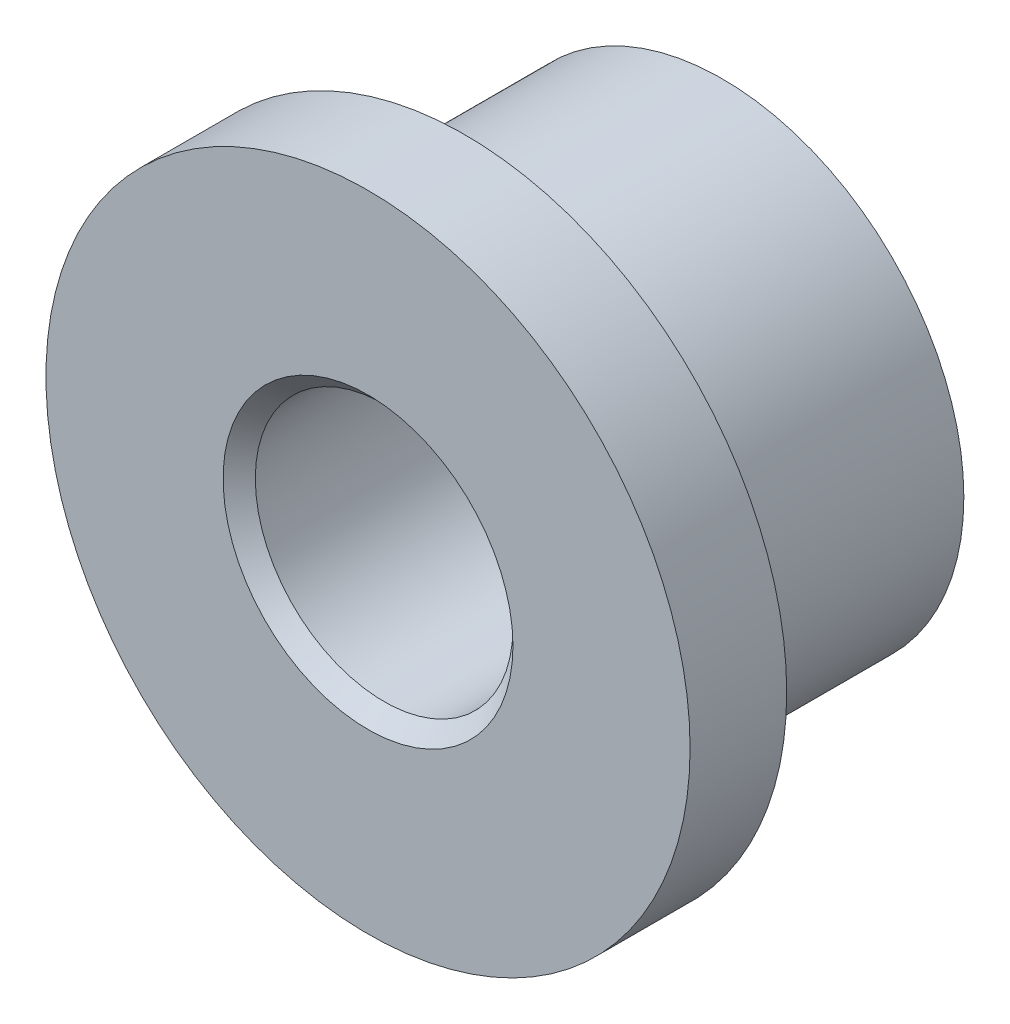
SolidWorks part; units mm, degrees
ref_plane "前视基准面" through (0, 0, 0) normal (0, 0, 1) x (1, 0, 0)
ref_plane "上视基准面" through (0, 0, 0) normal (0, 1, 0) x (1, 0, 0)
ref_plane "右视基准面" through (0, 0, 0) normal (1, 0, 0) x (0, 0, -1)
sketch "草图1" plane through (0, 0, 0) normal (0, 0, 1) x (1, 0, 0)
  circle A0 centre (145.5047, 180.5689) radius 7.5 construction
  circle A1 centre (145.5047, 180.5689) radius 7.5
  circle A2 centre (145.5047, 180.5689) radius 4
  dimension "D1" = 8
extrude "凸台-拉伸1" add sketch "草图1" against normal up to surface (8 mm away)
sketch "草图2" plane through (0, 0, 0) normal (0, 0, 1) x (1, 0, 0)
  circle A0 centre (145.5047, 180.5689) radius 4 construction
  circle A1 centre (145.5047, 180.5689) radius 4
  circle A2 centre (145.5047, 180.5689) radius 10
extrude "凸台-拉伸2" add sketch "草图2" along normal blind 3
chamfer "倒角1" distance 0.5 angle 45 2 edges at (149.5047, 180.5689, -8) (149.5047, 180.5689, 3)
